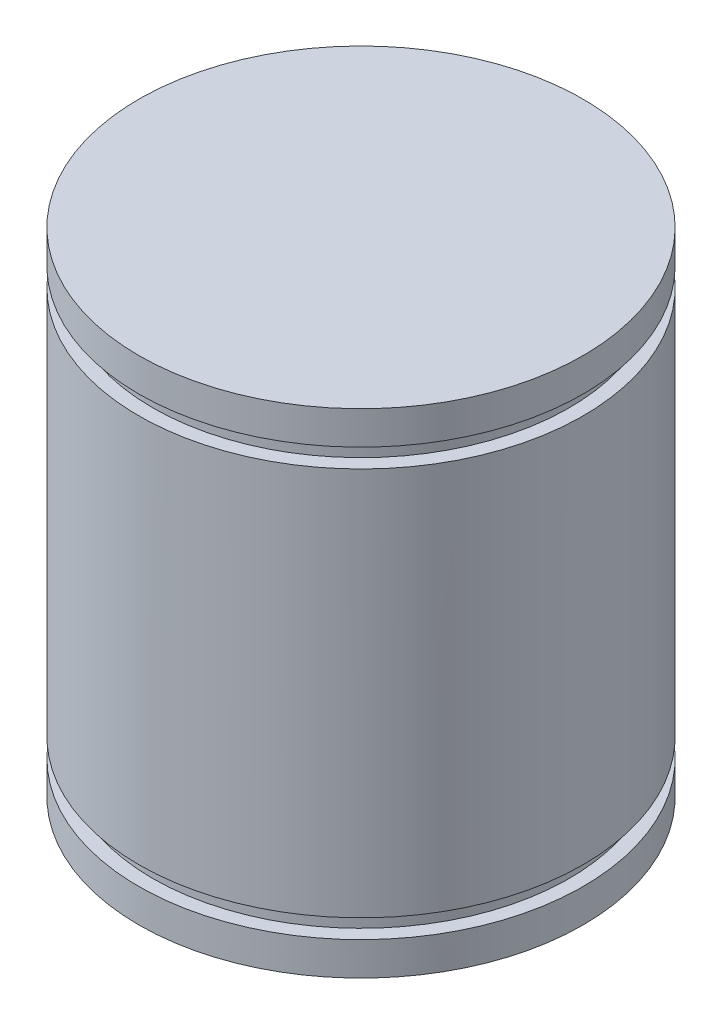
from build123d import *

# Parameters (mm, degrees)
SKETCH_1_R      = 20
EXTRUDE_1_DEPTH = 44.4
SKETCH_2_W      = 2.53960462
SKETCH_2_H      = 1.7


with BuildPart() as part:
    # 草图1 → 凸台-拉伸1 (new body)
    with BuildSketch(Plane(origin=(0, 0, 0), x_dir=(1, 0, 0), z_dir=(0, 1, 0))):
        with Locations(Location((0, 0, 0), (0, 0, 270))):
            Circle(SKETCH_1_R)
    extrude(amount=EXTRUDE_1_DEPTH)

    # 草图2 → 切除-旋转1 (revolve, cut)
    with BuildSketch(Plane.XY, mode=Mode.PRIVATE) as cut_revolve_1_sk:
        with Locations((-20.01980231, 3.85)):
            Rectangle(SKETCH_2_W, SKETCH_2_H)
    cut_revolve_1 = revolve(cut_revolve_1_sk.sketch.rotate(Axis((0, 44.4, 0), (0, -1, 0)), 270), axis=Axis((0, 44.4, 0), (0, -1, 0)), mode=Mode.SUBTRACT)

    # 镜向1: 切除-旋转1 across plane
    add(cut_revolve_1.mirror(Plane(origin=(0, 22.2, 0), x_dir=(0, 0, 1), z_dir=(0, -1, 0))), mode=Mode.SUBTRACT)


solid = part.part
